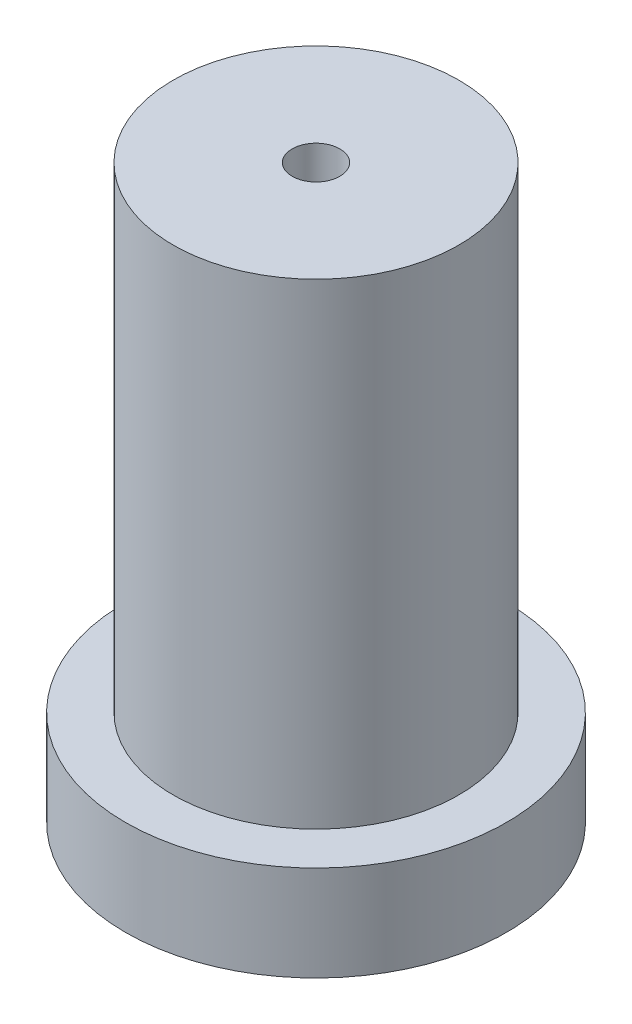
SolidWorks part; units mm, degrees
ref_plane "前视基准面" through (0, 0, 0) normal (0, 0, 1) x (1, 0, 0)
ref_plane "上视基准面" through (0, 0, 0) normal (0, 1, 0) x (1, 0, 0)
ref_plane "右视基准面" through (0, 0, 0) normal (1, 0, 0) x (0, 0, -1)
sketch "草图1" plane through (0, 0, 0) normal (0, 0, 1) x (1, 0, 0)
  line L0 (0, 0) -> (0, 4098.2049) construction
  line L1 (0.25, 3.7731) -> (0.25, -2.2269)
  line L2 (0.25, -2.2269) -> (2, -2.2269)
  line L3 (2, -2.2269) -> (2, -1.2269)
  line L4 (2, -1.2269) -> (1.5, -1.2269)
  line L5 (1.5, -1.2269) -> (1.5, 3.7731)
  line L6 (1.5, 3.7731) -> (0.25, 3.7731)
  dimension "D1" = 6
  dimension "D2" = 1.75
  dimension "D3" = 1
  dimension "D4" = 0.5
  dimension "D5" = 0.25
revolve "旋转1" add sketch "草图1" angle 360 about L0
